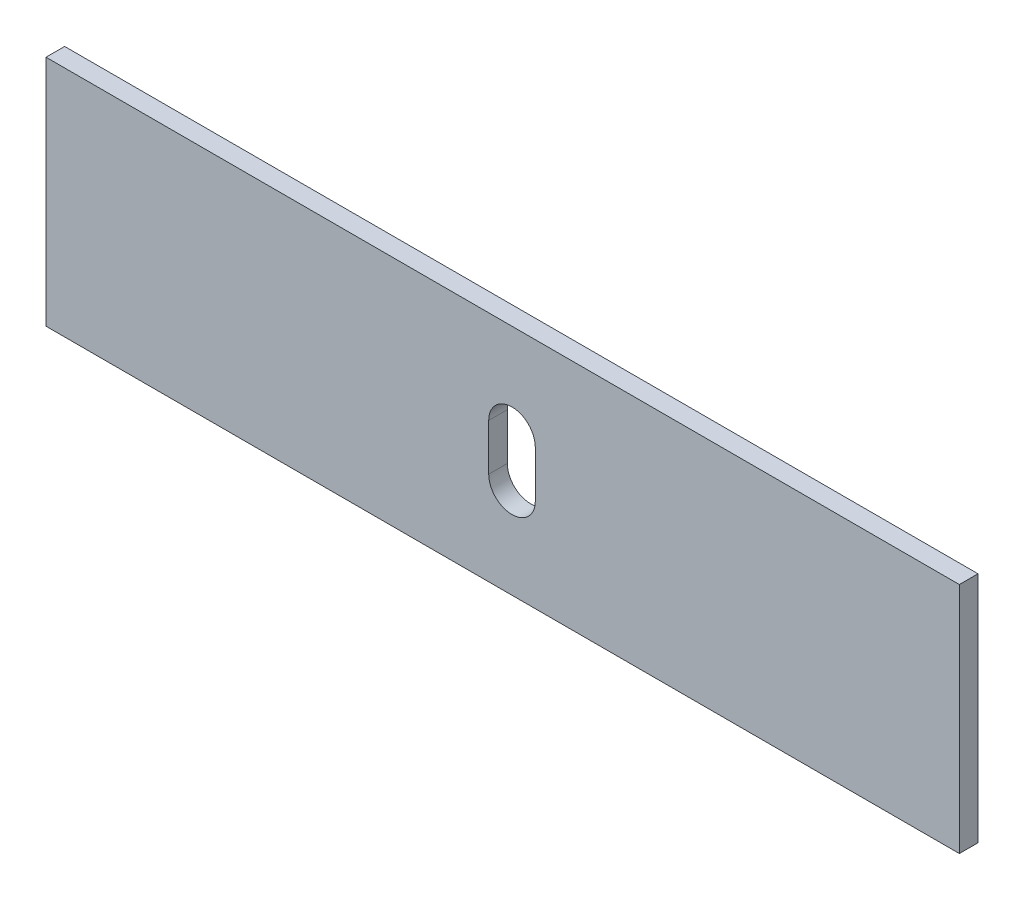
SolidWorks part; units mm, degrees
material "Q235B"
ref_plane "Front Plane" through (0, 0, 0) normal (0, 0, 1) x (1, 0, 0)
ref_plane "Top Plane" through (0, 0, 0) normal (0, 1, 0) x (1, 0, 0)
ref_plane "Right Plane" through (0, 0, 0) normal (1, 0, 0) x (0, 0, -1)
sketch "Sketch1" plane through (0, 0, 0) normal (0, 0, 1) x (1, 0, 0)
  line L0 (11341.1251, 4637.8242) -> (11341.1251, 4387.8242)
  line L1 (12321.1251, 4637.8242) -> (12321.1251, 4387.8242)
  line L2 (11341.1251, 4637.8242) -> (12321.1251, 4637.8242)
  line L3 (11341.1251, 4387.8242) -> (12321.1251, 4387.8242)
  line L4 (11816.1251, 4537.8242) -> (11816.1251, 4487.8242)
  line L5 (11866.1251, 4537.8236) -> (11866.1251, 4487.8244)
  arc A0 (11866.1251, 4537.8236) -> (11816.1251, 4537.8242) centre (11841.1251, 4537.8239) ccw
  arc A1 (11816.1251, 4487.8242) -> (11866.1251, 4487.8244) centre (11841.1251, 4487.8242) ccw
  dimension "D1" = 250
extrude "Boss-Extrude1" add sketch "Sketch1" along normal blind 20
